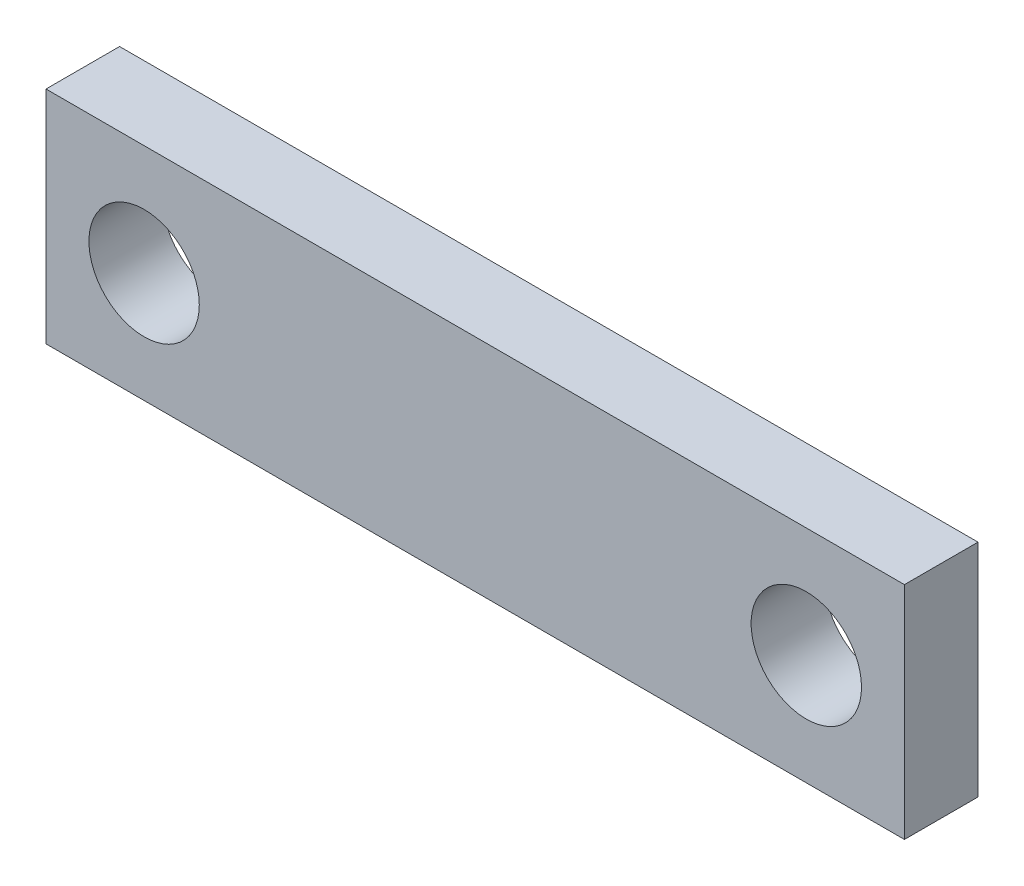
SolidWorks part; units mm, degrees
ref_plane "前视基准面" through (0, 0, 0) normal (0, 0, 1) x (1, 0, 0)
ref_plane "上视基准面" through (0, 0, 0) normal (0, 1, 0) x (1, 0, 0)
ref_plane "右视基准面" through (0, 0, 0) normal (1, 0, 0) x (0, 0, -1)
sketch "草图1" plane through (0, 0, 0) normal (0, 0, 1) x (1, 0, 0)
  line L1 (-17.5, -4.5) -> (17.5, -4.5)
  line L2 (-17.5, -4.5) -> (-17.5, 4.5)
  line L3 (-17.5, 4.5) -> (17.5, 4.5)
  line L4 (17.5, -4.5) -> (17.5, 4.5)
  line L5 (-17.5, -4.5) -> (17.5, 4.5) construction
  line L6 (-17.5, 4.5) -> (17.5, -4.5) construction
  circle A0 centre (-13.5, 0) radius 2.25
  circle A1 centre (13.5, 0) radius 2.25
  point P0 (0, 0)
  dimension "D3" = 4.5
  dimension "D1" = 35
  dimension "D2" = 9
  dimension "D4" = 4
  dimension "D5" = 4
extrude "凸台-拉伸1" add sketch "草图1" along normal mid plane 3
